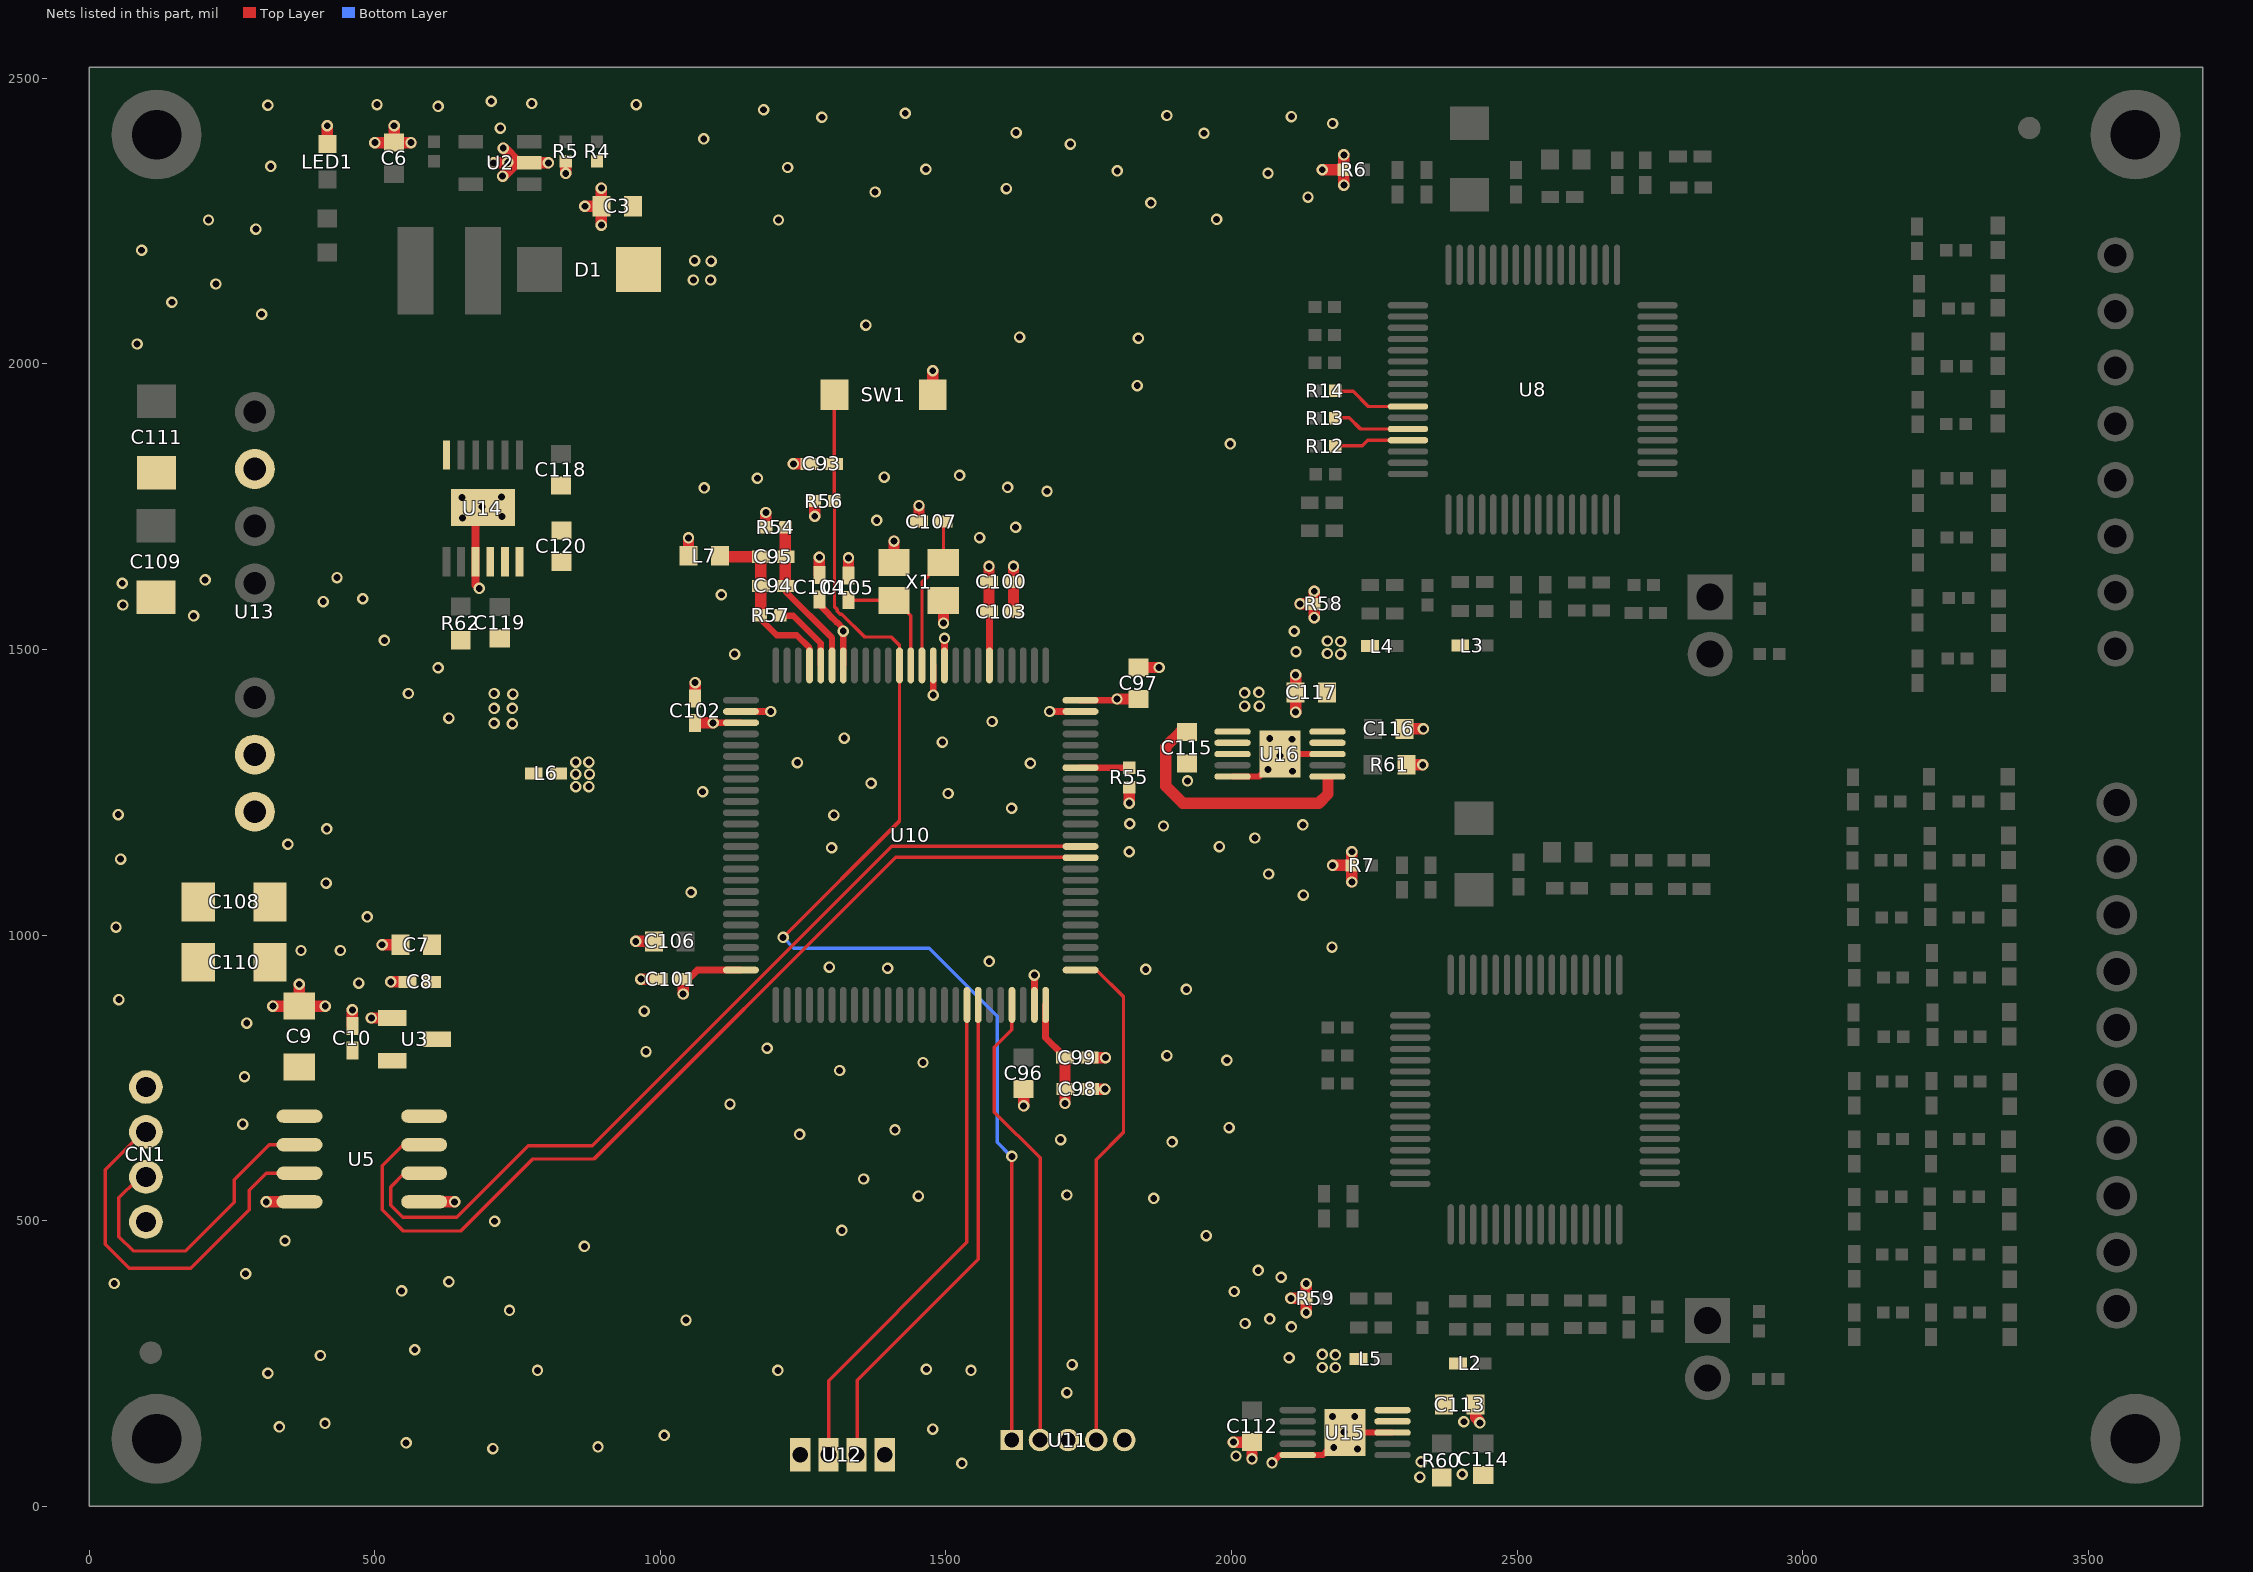
[diagram p0: the nets of this part, all layers, seen from the top]
# Altium PCB MISC86293.PcbDoc (part 4 of 4)
Units mil, origin at the board's own origin, x right, y up, seen from the top; angles counter-clockwise.
Board outline 3700.79 x 2519.68 mil, 4 copper layers (Top Layer, GND, POWER, Bottom Layer); 211 components, 128 nets, 717 pads, 581 vias.

## Via types
v1: diameter 20, hole 12, Top Layer to Bottom Layer, 581 vias

## Nets (pads, with @x,y where several pads share a name; then routed paths per layer and width w, separated by ;. In a path a pad name is that pad's centre, name@x,y a point inside that pad or via, vN(x,y) a via of type N, cw(c..) or ccw(c..) an arc to the next point about the centre after c; other vN are vias at no path point) (continued)
NetR12_1: R12.1 U8.45 | length 127.9
  Top Layer w6: R12.1@2185,1857 2229,1857 2238.42,1866.42 U8.45@2308.98,1866.42
NetR13_1: R13.1 U8.44 | length 132.2
  Top Layer w6: R13.1@2185,1906 2206,1906 2225.9,1886.1 U8.44@2308.98,1886.1
NetR14_1: R14.1 U8.42 | length 132
  Top Layer w6: R14.1@2188,1952 2213,1952 2239.53,1925.47 U8.42@2308.98,1925.47
NetR55_1: R55.1 U10.94 | length 85.4
  Top Layer w12: U10.94@1735.72,1293.11 R55.1@1821.11,1293.11
NetR57_2: R57.2 U10.21 | length 127.6
  Top Layer w11: R57.2@1212,1560 R57.2@1213,1560 ; R57.2@1213,1559 1233,1559 1281,1511 U10.21@1281,1472.24
OS_STM32_RX: CN1.3 U5.3 | length 655.6
  Top Layer w6: CN1.3@84,645 28,589 28,459 70,417 178,417 280,519 280,553 310,583 U5.3@368.33,583
OS_STM32_TX: CN1.2 U5.2 | length 539
  Top Layer w6: CN1.2@83,571 52,540 52,472 77,447 169,447 254,532 254,572 315,633 U5.2@368.33,633
OSC32_IN: C107.2 U10.12 X1.3 | length 244.1
  Top Layer w6: U10.12@1458.16,1472.24 1458.16,1618.16 X1.3@1480,1640 ; X1.3@1495.79,1652.47 C107.2@1495.79,1719.79
OSC32_OUT: C105.2 U10.13 X1.1 | length 187.1
  Top Layer w6: C105.2@1329.48,1586.54 X1.1@1414.46,1586.54 ; X1.1@1428,1570 1438.48,1559.52 U10.13@1438.48,1472.24
RAW_5V: C7.2 C8.2 C108.1 C110.1 CN1.1 U3.3 U13.2
RAW_STM32_RX: U5.6 U10.87 | length 1549.9
  Top Layer w6: U5.6@551,582 528,559 528,527 549,506 644,506 769,631 881,631 1405.31,1155.31 U10.87@1735.72,1155.31
RAW_STM32_TX: U5.7 U10.86 | length 1653
  Top Layer w6: U5.7@566,634 551,634 513,596 513,519 550,482 651,482 777,608 884,608 1412,1136 U10.86@1734,1136
RAW_VCC3V3: C9.1 C10.2 U3.2 U5.1
SIGNAL_GND: C3.1 C6.1 C93.1 C96.1 C97.1 C98.1 C99.1 C100.1 C101.1 C102.1 C103.1 C104.1 C105.1 C106.2 C107.1 C109.2 C111.2 C112.1 C113.2 C114.1 C115.1 C116.1 C117.2 C118.1 C119.1 C120.1 LED1.1 R5.1 R6.2 R7.2 R54.1 R55.2 R58.2 R59.2 R60.1 R61.2 R62.1 SW1.1 U2.2 U5.5 U10.10 U10.27 U10.74 U10.99 U11.3 U12.4 U13.7 U14.6 U14.9 U14.13 U15.5 U15.8 U15.11 U16.5 U16.8 U16.11 X1.2 X1.4 | length 2225.5
  Top Layer w11: U16.5@2001.93,1277.63 2048.63,1277.63 U16.11@2060,1289 ; v1(2071,76) 2084.63,89.63 U15.5@2115.93,89.63 2159.63,89.63 U15.11@2168,98 ; U16.11@2112,1317 U16.8@2168.07,1317 ; U15.11@2228,129 U15.8@2282.07,129
  Top Layer w12: U10.27@1141.24,1391.54 v1(1193.46,1391.54) ; U10.10@1497.54,1472.24 v1(1497.54,1519.54) ; U10.74@1655.02,877.76 v1(1655.02,930.02) ; v1(1681.54,1391.54) U10.99@1735.72,1391.54
  Top Layer w14: U14.13@676.72,1716.72 U14.9@676.72,1653.5 676.72,1613.28 v1(683,1607)
  Top Layer w20: LED1.1@416.99,2385.48 v1(416.99,2417) ; v1(500.44,2387.56) C6.1@534,2387.56 ; v1(534,2417) C6.1@534,2387.56 ; v1(563.56,2387.56) C6.1@534,2387.56 ; U5.5@586.63,533 v1(640,533) ; v1(708,2352) U2.2@770.67,2352 ; v1(724,2329) 747,2352 U2.2@770.67,2352 ; v1(725,2378) 751,2352 U2.2@770.67,2352 ; v1(804,2352) U2.2@770.67,2352 ; v1(834.48,2333.52) R5.1@834.48,2354.96 ; v1(868,2276) C3.1@896.92,2276 ; v1(896.92,2243.08) C3.1@896.92,2276 ; v1(896.92,2307.92) C3.1@896.92,2276 ; v1(957,989) C106.2@988.92,989 ; v1(966,923) C101.1@997.02,923 ; C102.1@1061,1414.46 v1(1061,1442) ; R54.1@1184.96,1714 v1(1184.96,1739.96) ; v1(1233,1825) C93.1@1261.02,1825 ; C104.1@1278.48,1630.46 v1(1278.48,1661.48) ; C105.1@1329.48,1629.46 v1(1329.48,1660.52) ; X1.4@1409.17,1652.47 v1(1409.17,1689.83) ; C107.1@1453.02,1724 v1(1453.02,1752.02) ; SW1.1@1477.02,1946 v1(1477.02,1987.98) ; v1(1495.79,1546.21) X1.2@1495.79,1585.53 ; C103.1@1618.46,1566.52 v1(1618.46,1645.46) ; v1(1636,701) C96.1@1636,730.44 ; C99.1@1751.46,785.48 v1(1779.48,785.48) ; C98.1@1752.46,730.48 v1(1778.48,730.48) ; v1(1821,1231) R55.2@1821,1258.96 ; C97.1@1837.48,1468.56 v1(1873.44,1468.56) ; v1(2003.44,112.44) C112.1@2036,112.44 v1(2036,83) ; v1(2104,364) R59.2@2130.96,364 ; v1(2112.44,1390.44) C117.2@2112.44,1425 v1(2112.44,1455.56) ; v1(2120,1580) R58.2@2144.96,1580 ; v1(2130.96,339.04) R59.2@2130.96,364 ; v1(2130.96,389.96) R59.2@2130.96,364 ; v1(2144.96,1555.96) R58.2@2144.96,1580 ; v1(2144.96,1601.96) R58.2@2144.96,1580 ; v1(2159,2340) R6.2@2196.96,2340 ; v1(2177,1122) R7.2@2210.96,1122 ; v1(2196.96,2313.04) R6.2@2196.96,2340 ; v1(2196.96,2366.04) R6.2@2196.96,2340 ; v1(2210.96,1092.96) R7.2@2210.96,1122 ; v1(2210.96,1145.96) R7.2@2210.96,1122 ; C116.1@2302.56,1361 v1(2336,1361) ; R61.2@2306.66,1298 v1(2335,1298) ; C113.2@2427.56,178 2427.56,155.44 v1@2434,149
  other v1: 2330,51 2404,56 1528,75 2332,78 2008,88 2221,100 707,101 2179,103 891,104 555,111 1007,124 2197,130 1477,135 333,139 413,145 2435,146 2407,148 2177,157 2216,157 1712,199 313,233 785,238 1206,238 1544,238 1466,240 1721,248 2101,260 405,264 570,274 2105,314 2024,320 1045,326 2067,328 736,343 2005,376 547,377 630,393 2087,401 2047,413 867,455 1956,474 1318,483 710,499 1864,539 1452,543 1712,545 1356,573 1896,638 1701,642 1244,651 1411,659 1996,663 1122,704 1314,763 1460,777 1992,781 1887,789 975,796 1187,802 972,867 1921,905 1850,940 1398,942 1296,944 1576,954 2176,979 2126,1070 1054,1075 2065,1107 1821,1146 1300,1153 1979,1155 2041,1170 1881,1191 2125,1193 1822,1195 1304,1210 1615,1222 1504,1248 1074,1251 1369,1266 1923,1270 2107,1287 2064,1290 1648,1301 1240,1302 2085,1314 1494,1338 2106,1343 2067,1344 1322,1345 1581,1374 630,1380 559,1423 611,1468 1130,1492 2113,1496 517,1516 2110,1532 183,1559 59,1578 410,1584 479,1589 1107,1596 58,1616 203,1622 434,1626 1559,1696 1622,1714 1379,1726 654,1730 723,1733 688,1750 653,1766 722,1767 1677,1777 1077,1783 1608,1784 1170,1800 1392,1802 1524,1805 1998,1860 1835,1962 84,2035 1837,2045 1629,2047 1360,2068 302,2087 145,2108 222,2140 92,2199 292,2236 209,2252 1207,2252 1974,2253 1859,2282 2134,2292 1376,2301 1606,2307 2064,2334 1800,2338 1465,2341 1223,2344 318,2346 733,2353 1718,2385 1076,2394 1952,2404 1623,2405 720,2413.02 2177,2421 1283,2432 2105,2433 1887,2435 1429,2439 1181,2445 611,2451 313,2453 504,2454 958,2454 775,2456 704,2460
STM32_AGND: C94.1 C95.1 R54.2 U10.20 | length 270.2
  Top Layer w11: C94.1@1220,1609 1220,1601 1300.68,1520.32 U10.20@1300.68,1472.24
  Top Layer w20: C94.1@1219.04,1613.96 R54.2@1219.04,1714
STM32_NRST: C93.2 R56.1 SW1.2 U10.14 U11.1 | length 2277
  Top Layer w6: v1(1215,996) 1418.79,1199.79 U10.14@1418.79,1472.24 1418.79,1507.21 1404,1522 1358,1522 1318.01,1561.99 1315.12,1561.99 1309.85,1567.26 1309.85,1570.15 1305,1575 R56.1@1305,1761 ; R56.1@1304.52,1760 SW1.2@1304.52,1928.52 ; U11.1@1615.58,116 v1(1615.58,612.58)
  Bottom Layer w6: v1(1215,996) 1234,977 1471,977 1590,858 1590,637 v1@1612,615 ; v1(1615.58,612.58) v1@1615.58,615
STM32_SWCLK: U10.76 U11.4 | length 886.5
  Top Layer w6: U10.76@1735.72,938.78 1764.22,938.78 1811,892 1811,655 1763,607 U11.4@1763,120
STM32_SWDIO: U10.72 U11.2 | length 796.6
  Top Layer w6: U10.72@1615.65,877.76 1615.65,834.65 1585,804 1585,690 1665,610 1665,149 U11.2@1665,127
STM32_UART1_RX: U10.69 U12.3 | length 867.4
  Top Layer w6: U12.3@1345,98 1345,221 1556.59,432.59 U10.69@1556.59,877.76
STM32_UART1_TX: U10.68 U12.2 | length 878
  Top Layer w6: U12.2@1295,100 1295,220 1536.91,461.91 U10.68@1536.91,877.76
STM_VCC3V3: C97.2 C98.2 C99.2 C100.2 C101.2 C102.2 C103.2 C104.2 L6.2 L7.1 R56.2 U10.6 U10.11 U10.19 U10.28 U10.50 U10.75 U10.100 U11.5 U12.1 | length 885.9
  Top Layer w11: C104.2@1279,1587 1279,1578 1295.35,1561.65 1295.35,1561.25 1309.12,1547.49 1309.51,1547.49 v1@1320.37,1536.63 ; U10.19@1320.37,1472.24 v1@1320.37,1536.63 ; v1(1320.37,1532.37) v1@1320.37,1536.63
  Top Layer w12: C101.2@1051,925 1064.78,938.78 U10.50@1141.24,938.78 ; v1@1096.15,1371.85 U10.28@1141.24,1371.85 ; v1(1477.85,1420.15) U10.11@1477.85,1472.24 ; U10.6@1576.28,1472.24 C103.2@1576.28,1560.72 ; U10.75@1674.7,877.76 1674.7,820.3 C99.2@1705,790 ; U10.100@1735.72,1411.22 v1@1796.78,1411.22
  Top Layer w20: v1(1039.94,896.94) C101.2@1039.94,923 ; L7.1@1049.44,1664 v1(1049.44,1695.56) ; C102.2@1061,1371.54 v1(1092.46,1371.54) ; v1(1270.44,1733.44) R56.2@1270.44,1760 ; C103.2@1575.54,1572.46 C100.2@1575.54,1618.52 v1(1575.54,1645.46) ; v1(1708.54,705.46) C99.2@1708.54,785.48 ; v1(1799.56,1413.44) C97.2@1837.48,1413.44
  other v1: 852,1260 875,1260 852,1282 876,1282 852,1303 875,1303
STM_VDDA: C94.2 C95.2 L7.2 R57.1 U10.22 | length 300.7
  Top Layer w11: R57.1@1176,1553 1204,1525 1239.08,1525 1261.31,1502.77 U10.22@1261.31,1472.24
  Top Layer w20: L7.2@1110.48,1662.52 C95.2@1176.54,1662.52 ; R57.1@1175.96,1560 C95.2@1175.96,1657.96
UGND: C7.1 C8.1 C9.2 C10.1 C108.2 C110.2 CN1.4 U3.1 U5.4 U13.1 | length 314.9
  Top Layer w20: v1(310,533) U5.4@368.33,533 ; v1(321.67,875.67) C9.2@368,875.67 ; v1(368,914) C9.2@368,875.67 ; v1(413.33,875.67) C9.2@368,875.67 ; C10.1@461,840.98 v1(461,869) ; v1(494.08,854.92) U3.1@530.63,854.92 ; v1(513,983) C7.1@545.44,983 ; v1(528,918) C8.1@557.54,918
  other v1: 44,390 274,407 343,465 269,669 272,752 276,846 52,887 472,916 371,973 440,973 47,1014 487,1032 415,1091 55,1133 348,1159 416,1186 51,1211
VCC3V3: C120.2 L4.1 L5.1 L6.1 U5.8 U14.10 U14.11 U14.12
  other v1: 2159,243 2182,243 2182,265 2159,266 741,1370 709,1371 709,1397 741,1397 742,1422 709,1423 2191,1492 2168,1493 2191,1514 2168,1515
VCC6V: C3.2 C115.2 D1.1 R4.2 U16.1 U16.2 U16.3 U16.6 | length 442.6
  Top Layer w20: C115.2@1922,1355.56 1910.56,1355.56 1885,1330 1885,1261 1915,1231 2153,1231 2169,1247 2169,1270
  other v1: 2023,1401 2049,1401 2023,1424 2048,1425 1058,2147 1088,2147 1089,2180 1060,2181
VDDA3V3: C113.1 L2.1 U15.9 U15.10
VDDA5V: C117.1 L3.1 U16.9 U16.10
pads on no net: U8.1 U8.3 U8.5 U8.7 U8.9 U8.11 U8.13 U8.15 U8.27 U8.29 U8.60 U8.64 U9.17 U9.18 U9.27 U9.29 U9.42 U9.44 U9.45 U9.46 U9.60 U9.64 U10.5 U10.7 U10.8 U10.9 U10.15 U10.16 U10.17 U10.18 U10.23 U10.24 U10.25 U10.29 U10.33 U10.34 U10.35 U10.36 U10.37 U10.43 U10.44 U10.45 U10.46 U10.47 U10.48 U10.51 U10.52 U10.53 U10.54 U10.55 U10.56 U10.57 U10.58 U10.59 U10.60 U10.61 U10.62 U10.63 U10.64 U10.65 U10.66 U10.67 U10.70 U10.71 U10.77 U10.78 U10.79 U10.80 U10.81 U10.82 U10.83 U10.84 U10.85 U10.88 U10.89 U10.90 U10.91 U10.92 U10.93 U10.95 U10.96 U10.97 U13.3 U13.5 U14.5 U15.4 U16.4

## Polygon pours and split planes (outlines as drawn)
EEG_DGND on Top Layer "Bottom Layer-No Net" (solid, remove dead copper, pour order 1024): 32 vertices, not listed, extent 2076,1458 2400,2213
EMG_DGND on Top Layer "Bottom Layer-No Net" (solid, remove dead copper, pour order 1023): 30 vertices, not listed, extent 2089,235 2425,914
EEG_AVSS on Top Layer "Bottom Layer-No Net" (solid, remove dead copper, pour order 1022): 44 vertices, not listed, extent 2235,1400 3665,2487
EMG_AVSS on Top Layer "Bottom Layer-No Net" (solid, remove dead copper, pour order 1021): 53 vertices, not listed, extent 2252,35 3664,1357
SIGNAL_GND on Top Layer "Bottom Layer-No Net" (solid, pour order 1020): 102 vertices, not listed, extent 42.25,34.86 2451.25,2486.86
STM_VCC3V3 on Top Layer "Bottom Layer-No Net" (solid, remove dead copper, pour order 1014): 19 vertices, not listed, extent 806,1248 889,1315
VCC3V3 on Top Layer "Bottom Layer-No Net" (solid, remove dead copper, pour order 1013): 17 vertices, not listed, extent 2155,1478 2258,1528
VCC3V3 on Top Layer "Bottom Layer-No Net" (solid, remove dead copper, pour order 1012): 2145,270 2145,241 2149,237 2155,231 2171,231 2230,231 2235,236 2239,240 2239,254 2239,267 2236,270 2230,276 2214,276 2151,276 2145,270
VCC6V on Top Layer "Bottom Layer-No Net" (solid, remove dead copper, pour order 1009): 34 vertices, not listed, extent 877,2109 1107,2366
NetD1_2 on Top Layer "Bottom Layer-No Net" (solid, remove dead copper, pour order 1008): 27 vertices, not listed, extent 654,2073 832,2327
RAW_VCC3V3 on Top Layer "Bottom Layer-No Net" (solid, remove dead copper, pour order 1006): 34 vertices, not listed, extent 327,670 557,814
EMG_AVDD on Top Layer "Bottom Layer-No Net" (solid, remove dead copper, pour order 1005): 35 vertices, not listed, extent 2423,218 2615,377
EMG_DVDD on Top Layer "Bottom Layer-No Net" (solid, remove dead copper, pour order 1003): 26 vertices, not listed, extent 2249,239 2350,379
EEG_AVDD on Top Layer "Bottom Layer-No Net" (solid, remove dead copper, pour order 1002): 34 vertices, not listed, extent 2428,1466 2620,1642
EEG_DVDD on Top Layer "Bottom Layer-No Net" (solid, remove dead copper, pour order 1000): 27 vertices, not listed, extent 2269,1489 2359,1629
DVCC_5V on Top Layer "Bottom Layer-No Net" (solid, remove dead copper, pour order 1000): 23 vertices, not listed, extent 1966,123 2148,217
VDDA3V3 on Top Layer "Bottom Layer-No Net" (solid, remove dead copper, pour order 1001): 30 vertices, not listed, extent 2250,143 2412,268
VCC6V on Top Layer "Bottom Layer-No Net" (solid, remove dead copper, pour order 1002): 28 vertices, not listed, extent 1901,1311 2059,1443
VDDA5V on Top Layer "Bottom Layer-No Net" (solid, remove dead copper, pour order 1003): 39 vertices, not listed, extent 2136,1331 2416,1523
VCC3V3 on Top Layer "Bottom Layer-No Net" (solid, remove dead copper, pour order 1004): 46 vertices, not listed, extent 546,671 877,1685
DVCC_5V on Top Layer "Bottom Layer-No Net" (solid, remove dead copper, pour order 1005): 94 vertices, not listed, extent 71,1622 860,2366
NetC111_1 on Top Layer "Bottom Layer-No Net" (solid, remove dead copper, pour order 1006): 20 vertices, not listed, extent 76,1880 330,1985
UGND on Top Layer "Bottom Layer-No Net" (solid, remove dead copper, pour order 1007): 20 vertices, not listed, extent 25,375 544,1261
RAW_5V on Top Layer "Bottom Layer-No Net" (solid, remove dead copper, pour order 1008): 54 vertices, not listed, extent 69,461 650,1361
SIGNAL_GND on Bottom Layer "Bottom Layer-No Net" (solid, remove dead copper, pour order 1032): 102 vertices, not listed, extent 42.11,33 2451.11,2485
EEG_DGND on Bottom Layer "Bottom Layer-No Net" (solid, remove dead copper, pour order 1031): 32 vertices, not listed, extent 2076,1458 2400,2213
EMG_DGND on Bottom Layer "Bottom Layer-No Net" (solid, remove dead copper, pour order 1030): 30 vertices, not listed, extent 2089,235 2425,914
EMG_AVSS on Bottom Layer "Bottom Layer-No Net" (solid, remove dead copper, pour order 1029): 53 vertices, not listed, extent 2252,35 3664,1357
EEG_AVSS on Bottom Layer "Bottom Layer-No Net" (solid, remove dead copper, pour order 1028): 44 vertices, not listed, extent 2235,1400 3665,2487
VCC6V on Bottom Layer "Bottom Layer-No Net" (solid, remove dead copper, pour order 1009): 35 vertices, not listed, extent 1022,1385 2068,2204
UGND on Bottom Layer "Bottom Layer-No Net" (solid, remove dead copper, pour order 1010): 20 vertices, not listed, extent 25,375 544,1260
DVCC_5V on Bottom Layer "Bottom Layer-No Net" (solid, remove dead copper, pour order 1011): 58 vertices, not listed, extent 399,163 2033,1902
SIGNAL_GND on GND (split plane): 96 vertices, not listed, extent 20.1,20.1 2473.91,2499.59
EMG_AVSS on GND (split plane): 39 vertices, not listed, extent 2243.09,20.1 3680.69,1369.91
EEG_AVSS on GND (split plane): 38 vertices, not listed, extent 2233.09,1390.09 3680.69,2499.59
UGND on GND (split plane): 458.91,1175 459.26,1172.39 460.26,1169.96 461.87,1167.87 587.91,1041.82 587.91,819.18 477.87,709.13 476.26,707.04 475.26,704.61 474.91,702 474.91,491.18 351.82,368.09 20.1,368.09 20.1,1251 458.91,1251
EEG_DGND on GND (split plane): 43 vertices, not listed, extent 2069.09,1439.09 2454.91,2265.24
EMG_DGND on GND (split plane): 23 vertices, not listed, extent 2079.09,226.09 2434.91,927.91
VCC3V3 on POWER (split plane): 29 vertices, not listed, extent 20.1,20.1 3680.69,2499.59
STM_VCC3V3 on POWER (split plane): 1914.91,1549.82 1914.91,20.1 769.09,20.1 769.09,1320.82 884.13,1435.87 885.74,1437.96 886.74,1440.39 887.09,1443 887.09,1698.82 977.18,1788.91 1675.82,1788.91
EMG_AVDD on POWER (split plane): 20 vertices, not listed, extent 2542.09,201.09 2816.91,1119.91
EEG_AVDD on POWER (split plane): 20 vertices, not listed, extent 2557.09,1455.09 2812.91,2347.91
EEG_DVDD on POWER (split plane): 2371.91,1924.82 2371.91,1538.18 2347.82,1514.09 2237.18,1514.09 2162.09,1589.18 2162.09,1653 2161.74,1655.61 2160.74,1658.04 2159.13,1660.13 2073.09,1746.18 2073.09,2100.82 2093.18,2120.91 2175.82,2120.91
EMG_DVDD on POWER (split plane): 2267.91,740.82 2267.91,506 2268.26,503.39 2269.26,500.96 2270.87,498.87 2345.91,423.82 2345.91,303.18 2313.82,271.09 2236.18,271.09 2108.09,399.18 2108.09,737.82 2139.18,768.91 2239.82,768.91

## Keep-outs
Keep-Out Layer:
  the board outline again, w5

## Other copper
GND (plane layer: these items are gaps in the copper):
  rectangle: -2,1251 481,1538
  lines w20: 4,1497 462,1497 469,1490 469,1175 598,1046 598,815 485,702 485,487 356,358 7,358 ; 2223,2511 2223,2279 2181,2237 2112,2237 2059,2184 2059,1679 2092,1646 2138,1646 2166,1618 2166,1472 2209,1429 2355,1429 2402,1382 2402,1299 2353,1250 2282,1250 2233,1201 2233,938 2195,900 2109,900 2069,860 2069,496 2153,412 2153,279 2216,216 2436,216 2484,168 2484,10 ; 2225,2279 2225,2278 2319,2184 2394,2184 2429,2149 2429,1812 2465,1776 2465,1716 2429,1680 2351,1680 2323,1652 2323,1440 ; 2237,938 2398,938 2445,891 2445,494 2371,420 2371,224 ; 2401,1380 3689,1380
POWER (plane layer: these items are gaps in the copper):
  lines w20: 759,1 759,1325 877,1443 877,1703 973,1799 1680,1799 1925,1554 1925,2 ; 2063,2105 2063,1742 2152,1653 2152,1585 2233,1504 2352,1504 2382,1534 2382,1929 2180,2131 2089,2131 2064,2106 ; 2098,743 2098,395 2232,261 2318,261 2356,299 2356,428 2278,506 2278,745 2244,779 2135,779 2099,743 ; 2532,263 2532,558 2635,661 2635,1104 2661,1130 2784,1130 2827,1087 2827,554 2733,460 2733,238 2686,191 2549,191 2532,208 2532,265 ; 2547,1512 2547,1603 2613,1669 2613,2310 2661,2358 2793,2358 2823,2328 2823,2072 2797,2046 2797,1543 2699,1445 2568,1445 2547,1466 2547,1517

## Silkscreen, mask and mechanical layers (free items; w line width, h text height)
Top Overlay:
  text "GND" at 217,729 h50
  text "RX" at 227,630 h50
  text "TX" at 226,562 h50
  text "5V" at 231,463 h50
  text "EEG_EMG_Module_V4.0" at 872,423 h100
  text "RX" at 1362,196 h50 r90
  text "TX" at 1314,194 h50 r90
  text "RST" at 1628,188 h50 r90
  text "SWCLK" at 1779,186 h50 r90
  text "GND" at 1407,185 h50 r90
  text "3V3" at 1258,184 h50 r90
  text "GND" at 1728,184 h50 r90
  text "3V3" at 1829,184 h50 r90
  text "SWDIO" at 1682,181 h50 r90
Bottom Overlay:
  text "EOGN" at 3432,2177 h50
  text "EOGP" at 3432,2074 h50
  text "FZ" at 3432,1978 h50
  text "CZ" at 3432,1874 h50
  text "A1" at 3432,1783 h50
  text "PZ" at 3432,1677 h50
  text "REF" at 3432,1579 h50
  text "BIAS" at 3431,1475 h50
  text "C1" at 3432,1217 h50
  text "C2" at 3431,1114 h50
  text "C4" at 3431,1013 h50
  text "C3" at 3431,919 h50
  text "V1" at 3431,820 h50
  text "V2" at 3431,723 h50
  text "V3" at 3431,623 h50
  text "V4" at 3431,524 h50
  text "RA" at 3431,425 h50
  text "RL" at 3430,328 h50